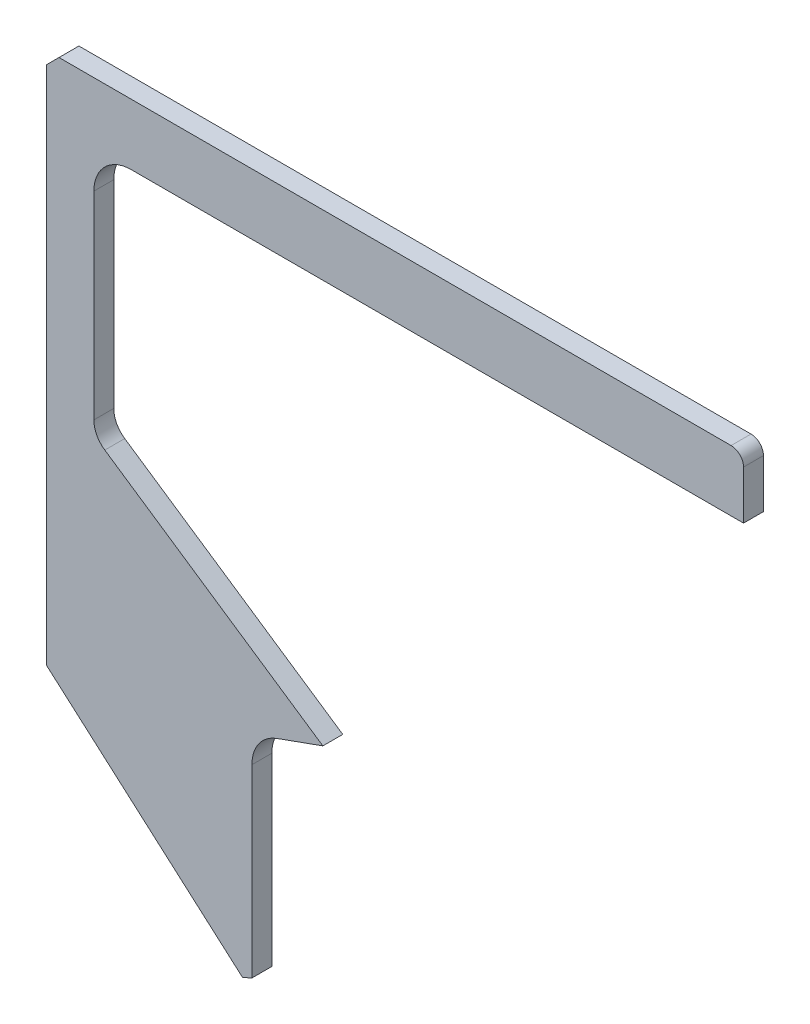
SolidWorks part; units mm, degrees
ref_plane "Front Plane" through (0, 0, 0) normal (0, 0, 1) x (1, 0, 0)
ref_plane "Top Plane" through (0, 0, 0) normal (0, 1, 0) x (1, 0, 0)
ref_plane "Right Plane" through (0, 0, 0) normal (1, 0, 0) x (0, 0, -1)
sketch "Sketch1" plane through (0, 0, 0) normal (0, 0, 1) x (1, 0, 0)
  line L0 (0, 145) -> (0, 563)
  line L1 (10, 573) -> (550, 573)
  line L2 (560, 563) -> (560, 524)
  line L3 (560, 524) -> (68, 524)
  line L4 (38, 494) -> (38, 334.8299)
  line L5 (46.8105, 318.2529) -> (222, 200)
  line L6 (222, 200) -> (184.8472, 186.638)
  line L7 (165, 158.4082) -> (165, 10)
  line L8 (157.4884, 6.6011) -> (0, 145)
  line L9 (0, 563) -> (10, 573)
  line L10 (165, 10) -> (157.4884, 6.6011)
  arc A0 (560, 563) -> (550, 573) centre (550, 563) ccw
  arc A1 (38, 334.8299) -> (46.8105, 318.2529) centre (58, 334.8299) ccw
  arc A2 (184.8472, 186.638) -> (165, 158.4082) centre (195, 158.4082) ccw
  arc A3 (68, 524) -> (38, 494) centre (68, 494) ccw
  point P1 (0, 573)
  point P10 (165, 0)
  point P12 (560, 573)
  point P19 (38, 324.2)
  point P22 (165, 179.5)
  dimension "D11" = 10
  dimension "D13" = 20
  dimension "D15" = 30
  dimension "D17" = 30
  dimension "D1" = 560
  dimension "D2" = 49
  dimension "D3" = 573
  dimension "D4" = 38
  dimension "D5" = 248.8
  dimension "D6" = 222
  dimension "D7" = 200
  dimension "D8" = 179.5
  dimension "D9" = 165
  dimension "D10" = 145
  dimension "D12" = 573
extrude "Boss-Extrude1" add sketch "Sketch1" along normal blind 16
